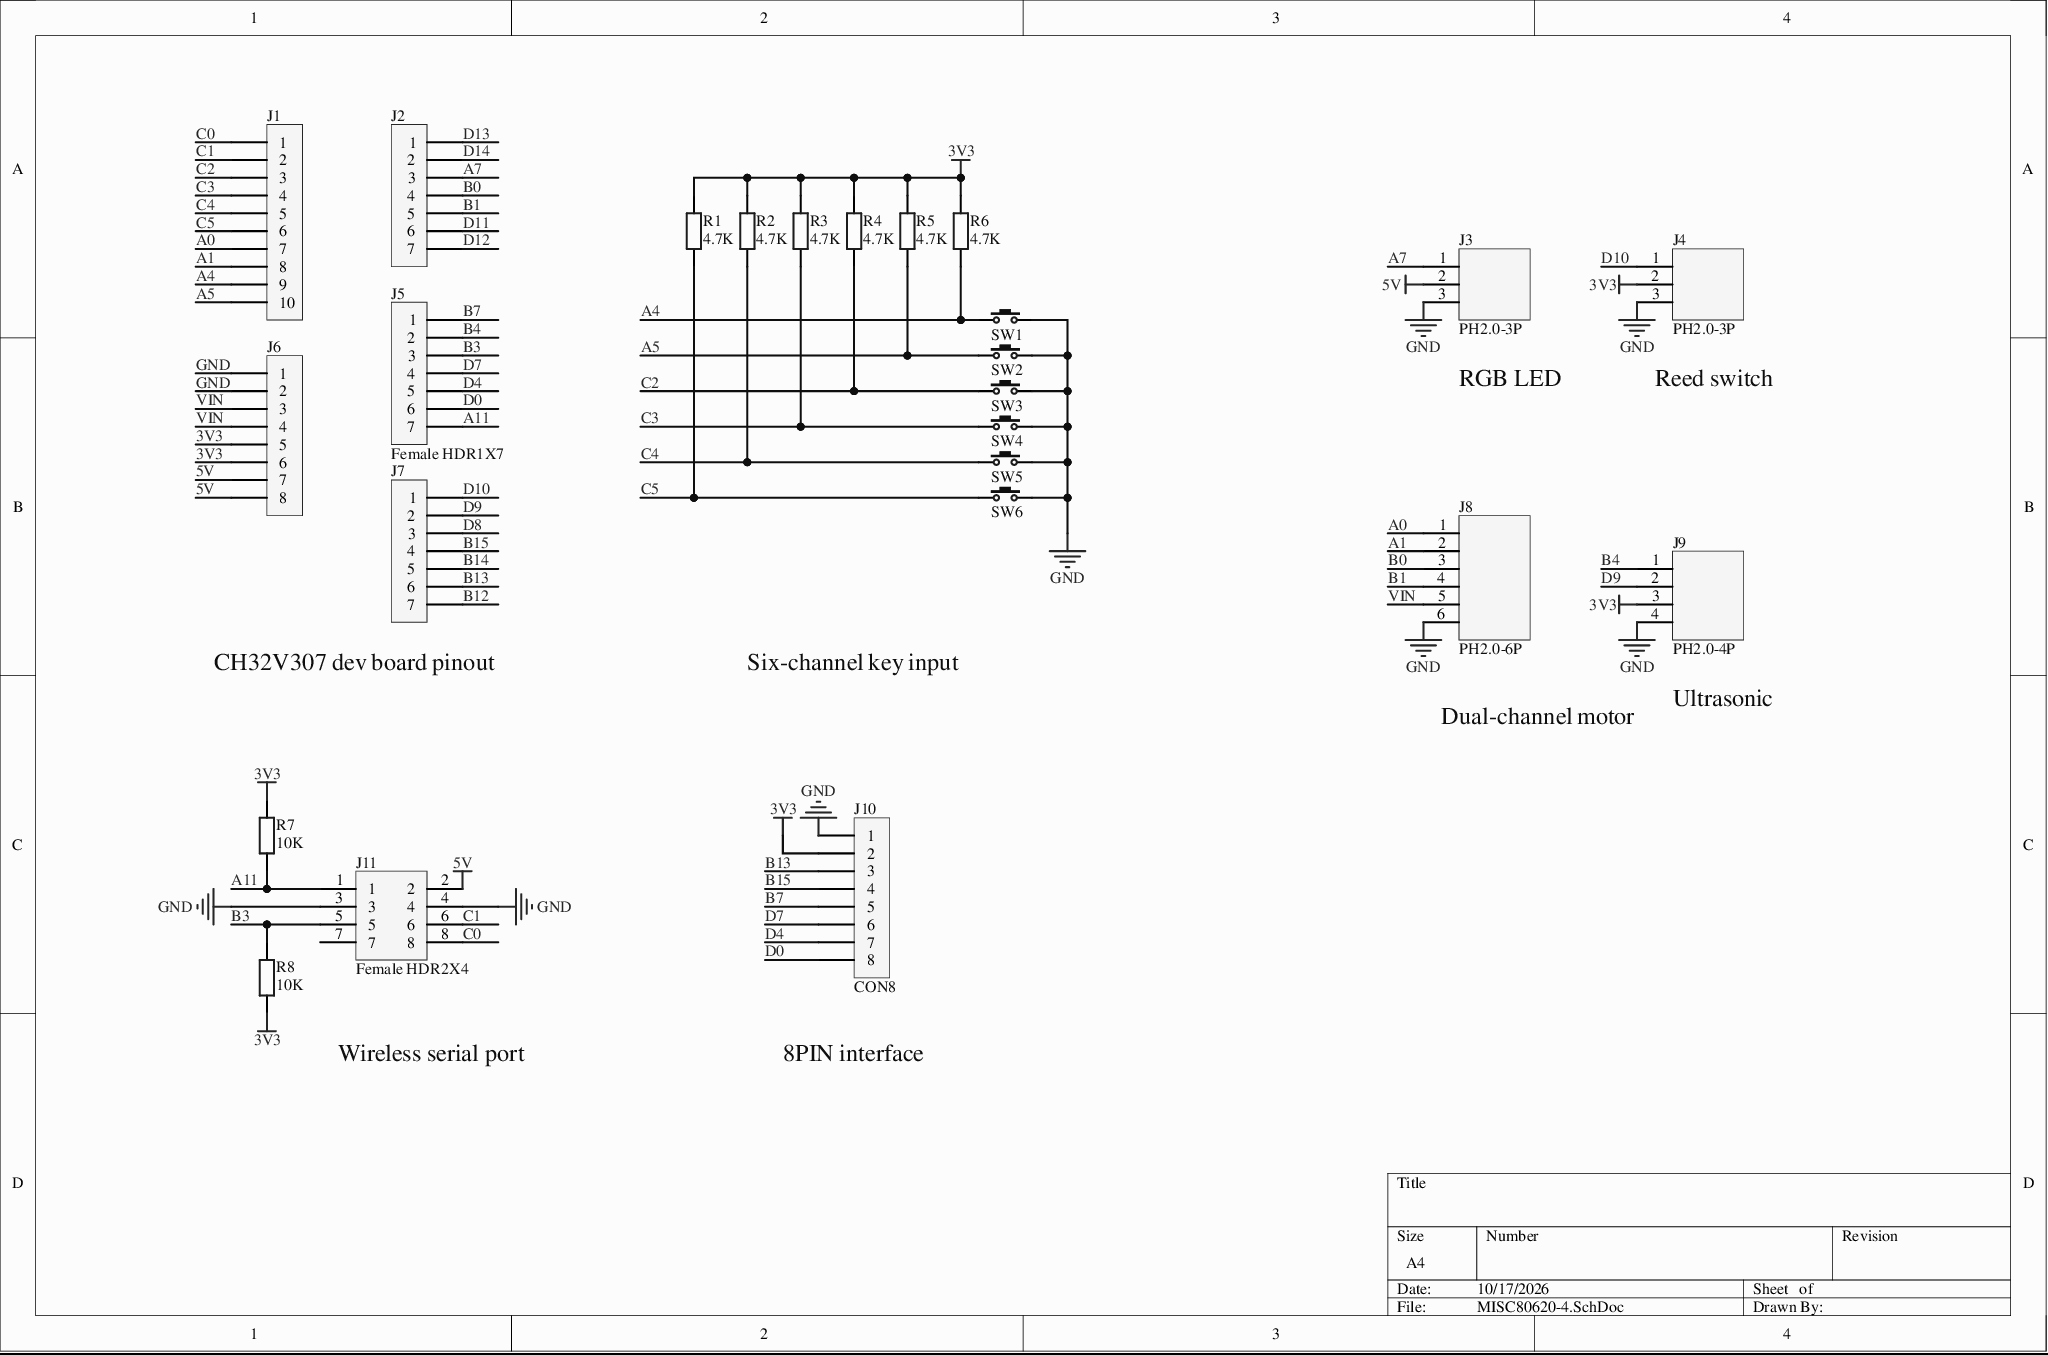
[diagram p0: MISC80620-4.SchDoc]
# Altium project MISC80620-7.PrjPcb
1 sheet, 25 parts. Net scope: global (net labels, ports and power ports of the same name join across sheets).
Board file: MISC80620.PcbDoc

## Sheet MISC80620-4.SchDoc
size A4

### Parts
J1  Female HDR1X10  [Fe-HDR1X10/2.54-S]  (value not drawn)
J2  Female HDR1X7  [Fe-HDR1X7/2.54-S]  (value not drawn)
J3  PH2.0-3P  [PH2.0-3P]
J4  PH2.0-3P  [PH2.0-3P]
J5  Female HDR1X7  [Fe-HDR1X7/2.54-S]
J6  Female HDR1X8  [Fe-HDR1X8/2.54-S]  (value not drawn)
J7  Female HDR1X7  [Fe-HDR1X7/2.54-S]  (value not drawn)
J8  PH2.0-6P  [PH2.0-6P]
J9  PH2.0-4P  [PH2.0-4P]
J10  CON8  [Fe-HDR1X8/2.54-S]
J11  Female HDR2X4  [Fe-HDR2X4/2.54-S]
R1  4.7K  [R 0805_L]
R2  4.7K  [R 0805_L]
R3  4.7K  [R 0805_L]
R4  4.7K  [R 0805_L]
R5  4.7K  [R 0805_L]
R6  4.7K  [R 0805_L]
R7  10K  [R 0805_L]
R8  10K  [R 0805_L]
SW1  3x6x5  [TSW DIP-3*6*4.3]  (value not drawn)
SW2  3x6x5  [TSW DIP-3*6*4.3]  (value not drawn)
SW3  3x6x5  [TSW DIP-3*6*4.3]  (value not drawn)
SW4  3x6x5  [TSW DIP-3*6*4.3]  (value not drawn)
SW5  3x6x5  [TSW DIP-3*6*4.3]  (value not drawn)
SW6  3x6x5  [TSW DIP-3*6*4.3]  (value not drawn)

### Nets
3V3: J4.2 J6.5 J6.6 J9.3 J10.2 R1.2 R2.2 R3.2 R4.2 R5.2 R6.2 R7.2 R8.1
5V: J3.2 J6.7 J6.8 J11.2
GND: J3.3 J4.3 J6.1 J6.2 J8.6 J9.4 J10.1 J11.3 J11.4 SW1.2 SW2.2 SW3.2 SW4.2 SW5.2 SW6.2
A0: J1.7 J8.1
A1: J1.8 J8.2
A4: J1.9 R6.1 SW1.1
A5: J1.10 R5.1 SW2.1
A7: J2.3 J3.1
A11: J5.7 J11.1 R7.1
B0: J2.4 J8.3
B1: J2.5 J8.4
B3: J5.3 J11.5 R8.2
B4: J5.2 J9.1
B7: J5.1 J10.5
B12: J7.7
B13: J7.6 J10.3
B14: J7.5
B15: J7.4 J10.4
C0: J1.1 J11.8
C1: J1.2 J11.6
C2: J1.3 R4.1 SW3.1
C3: J1.4 R3.1 SW4.1
C4: J1.5 R2.1 SW5.1
C5: J1.6 R1.1 SW6.1
D0: J5.6 J10.8
D4: J5.5 J10.7
D7: J5.4 J10.6
D8: J7.3
D9: J7.2 J9.2
D10: J4.1 J7.1
D11: J2.6
D12: J2.7
D13: J2.1
D14: J2.2
VIN: J6.3 J6.4 J8.5

Not connected (* = marked no-connect by the designer): J11 7

### Notes on the sheet
- (near J3) RGB LED
- (near J4) Reed switch
- (near J7) CH32V307 dev board pinout
- Six-channel key input
- Dual-channel motor
- (near J9) Ultrasonic
- Wireless serial port
- 8PIN interface

### Library data of the parts
J10 = Female HDR1X8
R1-R8 = R: SMD resistor; BOM名称: SMD resistor
SW1-SW6 = TSW 3x6: 3x6 tact switch; BOM名称: 3x6 tact switch